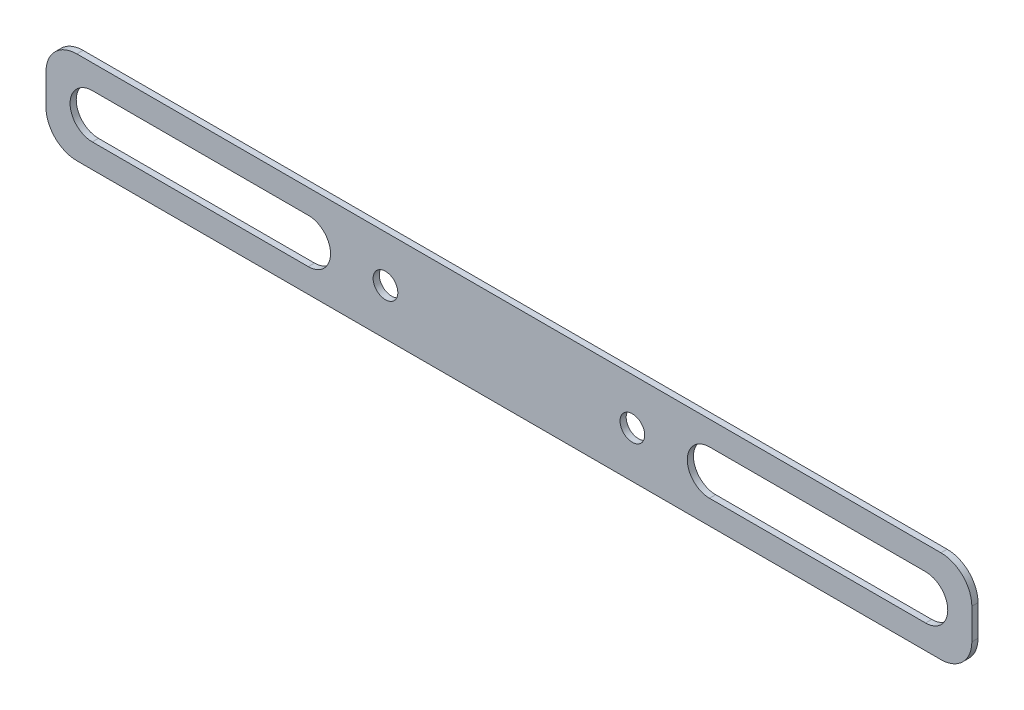
SolidWorks part; units mm, degrees
ref_plane "Front Plane" through (0, 0, 0) normal (0, 0, 1) x (1, 0, 0)
ref_plane "Top Plane" through (0, 0, 0) normal (0, 1, 0) x (1, 0, 0)
ref_plane "Right Plane" through (0, 0, 0) normal (1, 0, 0) x (0, 0, -1)
sketch "Sketch1" plane through (0, 0, 0) normal (0, 0, 1) x (1, 0, 0)
  line L1 (150, -15) -> (-150, -15)
  line L2 (150, -15) -> (150, 15)
  line L3 (150, 15) -> (-150, 15)
  line L4 (-150, -15) -> (-150, 15)
  line L5 (150, -15) -> (-150, 15) construction
  line L6 (150, 15) -> (-150, -15) construction
  point P0 (0, 0)
  dimension "D1" = 300
  dimension "D2" = 30
extrude "Boss-Extrude1" add sketch "Sketch1" along normal blind 2
sketch "Sketch2" plane through (0, 0, 2) normal (0, 0, 1) x (1, 0, 0)
  line L0 (-135, 0) -> (-65, 0) construction
  line L1 (-135, 7.2) -> (-65, 7.2)
  line L2 (-135, -7.2) -> (-65, -7.2)
  arc A0 (-135, 7.2) -> (-135, -7.2) centre (-135, 0) ccw
  arc A1 (-65, -7.2) -> (-65, 7.2) centre (-65, 0) ccw
  point P3 (-100, 0)
  dimension "D2" = 7.2
  dimension "D1" = 70
  dimension "D3" = 100
extrude "Cut-Extrude1" cut sketch "Sketch2" against normal through all
fillet "Fillet1" radius 10 2 edges at (-150, 15, 1) (-150, -15, 1)
mirror "Mirror1" about plane through (0, 0, 0) normal (1, 0, 0) of "Cut-Extrude1"
fillet "Fillet2" radius 10 2 edges at (150, -15, 1) (150, 15, 1)
sketch "Sketch4" plane through (0, 0, 0) normal (0, 0, -1) x (-1, 0, 0)
  circle A0 centre (40, 0) radius 4
  circle A1 centre (-40, 0) radius 4
  dimension "D1" = 40
  dimension "D2" = 8
  dimension "D3" = 80
extrude "Cut-Extrude2" cut sketch "Sketch4" against normal through all
